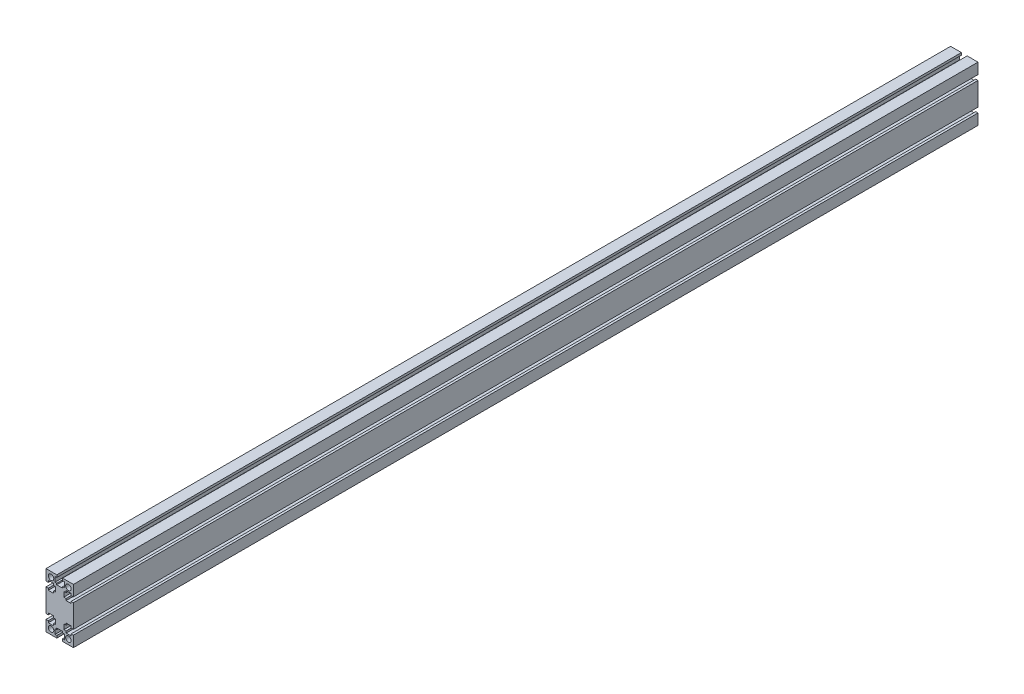
SolidWorks part; units mm, degrees
ref_plane "前视基准面" through (0, 0, 0) normal (0, 0, 1) x (1, 0, 0)
ref_plane "上视基准面" through (0, 0, 0) normal (0, 1, 0) x (1, 0, 0)
ref_plane "右视基准面" through (0, 0, 0) normal (1, 0, 0) x (0, 0, -1)
sketch "草图1" plane through (0, 0, 0) normal (0, 0, 1) x (1, 0, 0)
  line L0 (-27.4957, 11.1925) -> (-24.9957, 11.1925)
  line L1 (-27.4957, 23.0425) -> (-15.6457, 23.0425)
  line L2 (-27.4957, 23.0425) -> (-27.4957, 11.1925)
  line L3 (-27.4957, -36.9575) -> (-15.6457, -36.9575)
  line L4 (2.5043, 23.0425) -> (2.5043, 11.1925)
  line L5 (-24.9957, 11.1925) -> (-24.9957, 13.1925)
  line L6 (-24.9957, 13.1925) -> (-19.4957, 13.1925)
  line L7 (-19.4957, 13.1925) -> (-19.4957, 11.1925)
  line L14 (-24.9957, 5.6925) -> (-27.4957, 5.6925)
  line L15 (-27.4957, 5.6925) -> (-27.4957, -19.6075)
  line L18 (-19.4957, 5.6925) -> (-16.9957, 5.6925)
  line L19 (-16.9957, 5.6925) -> (-16.9957, 11.1925)
  line L20 (-16.9957, 11.1925) -> (-19.4957, 11.1925)
  line L21 (-24.9957, 5.6925) -> (-24.9957, 3.6925)
  line L22 (-24.9957, 3.6925) -> (-19.4957, 3.6925)
  line L23 (-19.4957, 3.6925) -> (-19.4957, 5.6925)
  line L24 (-12.4957, 23.0425) -> (-12.4957, 50023.0425) construction
  line L25 (0.0043, 5.6925) -> (2.5043, 5.6925)
  line L26 (0.0043, 5.6925) -> (0.0043, 3.6925)
  line L27 (0.0043, 3.6925) -> (-5.4957, 3.6925)
  line L28 (-5.4957, 3.6925) -> (-5.4957, 5.6925)
  line L29 (-5.4957, 5.6925) -> (-7.9957, 5.6925)
  line L30 (-7.9957, 5.6925) -> (-7.9957, 11.1925)
  line L31 (-7.9957, 11.1925) -> (-5.4957, 11.1925)
  line L32 (-5.4957, 13.1925) -> (-5.4957, 11.1925)
  line L33 (2.5043, 11.1925) -> (0.0043, 11.1925)
  line L34 (0.0043, 11.1925) -> (0.0043, 13.1925)
  line L35 (0.0043, 13.1925) -> (-5.4957, 13.1925)
  line L36 (2.5043, 5.6925) -> (2.5043, -19.6075)
  line L37 (-15.6457, 23.0425) -> (-15.6457, 20.5425)
  line L38 (-15.6457, 20.5425) -> (-17.6457, 20.5425)
  line L39 (-17.6457, 20.5425) -> (-17.6457, 15.0425)
  line L40 (-17.6457, 15.0425) -> (-15.7481, 15.0425)
  line L41 (-15.7481, 15.0425) -> (-15.7481, 13.5076)
  line L42 (-15.7481, 13.5076) -> (-9.2434, 13.5076)
  line L43 (-9.3457, 23.0425) -> (2.5043, 23.0425)
  line L45 (-9.2434, 15.0425) -> (-9.2434, 13.5076)
  line L46 (-7.3457, 15.0425) -> (-9.2434, 15.0425)
  line L47 (-9.3457, 20.5425) -> (-7.3457, 20.5425)
  line L48 (-7.3457, 20.5425) -> (-7.3457, 15.0425)
  line L49 (-9.3457, 23.0425) -> (-9.3457, 20.5425)
  line L50 (-9.3457, -36.9575) -> (-9.3457, -34.4575)
  line L51 (-9.3457, -34.4575) -> (-7.3457, -34.4575)
  line L52 (48.9171, -6.9575) -> (-49951.0829, -6.9575) construction
  line L53 (-7.3457, -34.4575) -> (-7.3457, -28.9575)
  line L54 (-7.3457, -28.9575) -> (-9.2434, -28.9575)
  line L55 (-9.2434, -28.9575) -> (-9.2434, -27.4226)
  line L56 (-5.4957, -27.1075) -> (-5.4957, -25.1075)
  line L57 (0.0043, -27.1075) -> (-5.4957, -27.1075)
  line L58 (0.0043, -25.1075) -> (0.0043, -27.1075)
  line L59 (2.5043, -25.1075) -> (0.0043, -25.1075)
  line L60 (0.0043, -19.6075) -> (2.5043, -19.6075)
  line L61 (0.0043, -19.6075) -> (0.0043, -17.6075)
  line L62 (-5.4957, -17.6075) -> (-5.4957, -19.6075)
  line L63 (0.0043, -17.6075) -> (-5.4957, -17.6075)
  line L64 (-5.4957, -19.6075) -> (-7.9957, -19.6075)
  line L65 (-7.9957, -19.6075) -> (-7.9957, -25.1075)
  line L66 (-7.9957, -25.1075) -> (-5.4957, -25.1075)
  line L67 (-15.7481, -27.4226) -> (-9.2434, -27.4226)
  line L68 (-15.7481, -28.9575) -> (-15.7481, -27.4226)
  line L69 (-17.6457, -28.9575) -> (-15.7481, -28.9575)
  line L70 (-15.6457, -36.9575) -> (-15.6457, -34.4575)
  line L71 (-15.6457, -34.4575) -> (-17.6457, -34.4575)
  line L72 (-17.6457, -34.4575) -> (-17.6457, -28.9575)
  line L73 (-24.9957, -27.1075) -> (-19.4957, -27.1075)
  line L74 (-19.4957, -27.1075) -> (-19.4957, -25.1075)
  line L75 (-16.9957, -25.1075) -> (-19.4957, -25.1075)
  line L76 (-16.9957, -19.6075) -> (-16.9957, -25.1075)
  line L77 (-19.4957, -19.6075) -> (-16.9957, -19.6075)
  line L78 (-19.4957, -17.6075) -> (-19.4957, -19.6075)
  line L79 (-24.9957, -17.6075) -> (-19.4957, -17.6075)
  line L80 (-24.9957, -19.6075) -> (-24.9957, -17.6075)
  line L81 (-24.9957, -25.1075) -> (-24.9957, -27.1075)
  line L82 (-27.4957, -25.1075) -> (-24.9957, -25.1075)
  line L83 (-24.9957, -19.6075) -> (-27.4957, -19.6075)
  line L84 (-27.4957, -25.1075) -> (-27.4957, -36.9575)
  line L85 (2.5043, -25.1075) -> (2.5043, -36.9575)
  line L86 (-9.3457, -36.9575) -> (2.5043, -36.9575)
  circle A0 centre (-21.9957, 17.5425) radius 3
  circle A1 centre (-2.9957, 17.5425) radius 3
  circle A2 centre (-2.9957, -31.4575) radius 3
  circle A3 centre (-21.9957, -31.4575) radius 3
  point P43 (-12.4957, 13.5076)
  dimension "D14" = 6
  dimension "D1" = 60
  dimension "D2" = 30
  dimension "D3" = 11.85
  dimension "D4" = 2.5
  dimension "D5" = 2
  dimension "D6" = 5.5
  dimension "D7" = 2
  dimension "D8" = 2.5
  dimension "D9" = 5.5
  dimension "D10" = 2.5
  dimension "D11" = 2
  dimension "D12" = 2
  dimension "D13" = 5.5
  dimension "D15" = 5.5
  dimension "D16" = 5.5
  dimension "D17" = 6.3
  dimension "D18" = 2.5
  dimension "D19" = 2
  dimension "D20" = 5.5
  dimension "D21" = 1.8977
extrude "凸台-拉伸1" add sketch "草图1" along normal blind 990
